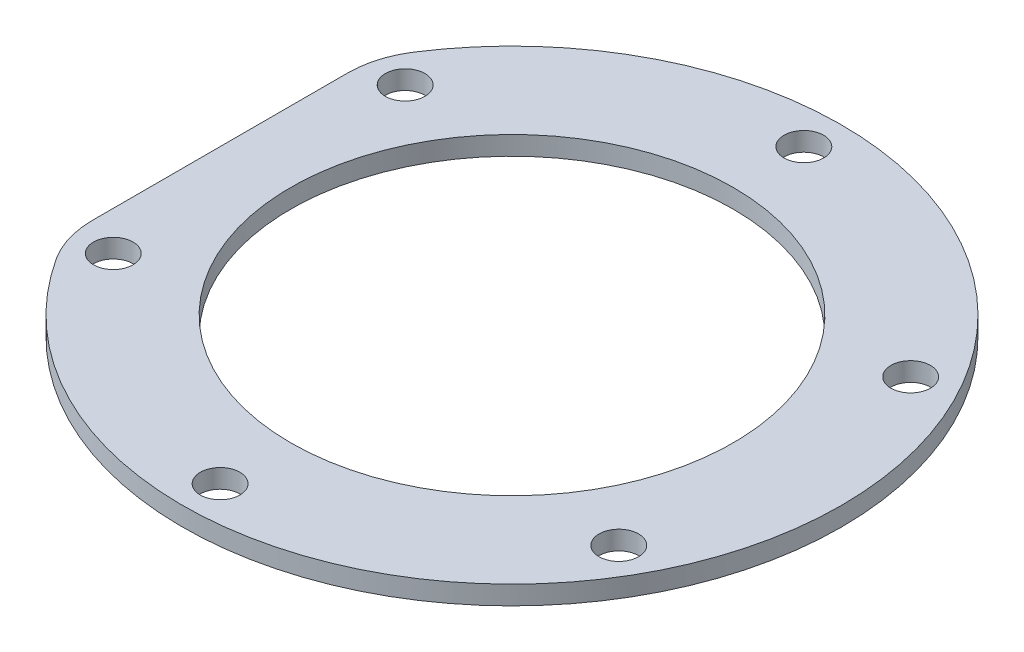
from build123d import *

# Parameters (mm, degrees)
SKETCH_1_R      = 23.5
SKETCH_1_R_2    = 2.1
EXTRUDE_1_DEPTH = 2


with BuildPart() as part:
    # 草图1 → 凸台-拉伸1 (new body)
    with BuildSketch(Plane(origin=(0, 0, 0), x_dir=(1, 0, 0), z_dir=(0, 1, 0))):
        with BuildLine():
            Line((-31, -13.564659966), (-31, 13.564659966))
            ThreePointArc((-31, 13.564659966), (-30.591663047, 16.393087091), (-29.4, 18.990523953))
            ThreePointArc((-29.4, 18.990523953), (35, 0), (-29.4, -18.990523953))
            ThreePointArc((-29.4, -18.990523953), (-30.591663047, -16.393087091), (-31, -13.564659966))
        make_face()
        with Locations(Location((0, 0, 0), (0, 0, 270))):
            Circle(SKETCH_1_R, mode=Mode.SUBTRACT)
        with Locations(Location((0, 31, 0), (0, 0, 270))):
            Circle(SKETCH_1_R_2, mode=Mode.SUBTRACT)
        with Locations(Location((26.846787517, 15.5, 0), (0, 0, 270))):
            Circle(SKETCH_1_R_2, mode=Mode.SUBTRACT)
        with Locations(Location((26.846787517, -15.5, 0), (0, 0, 270))):
            Circle(SKETCH_1_R_2, mode=Mode.SUBTRACT)
        with Locations(Location((0, -31, 0), (0, 0, 270))):
            Circle(SKETCH_1_R_2, mode=Mode.SUBTRACT)
        with Locations(Location((-26.846787517, -15.5, 0), (0, 0, 270))):
            Circle(SKETCH_1_R_2, mode=Mode.SUBTRACT)
        with Locations(Location((-26.846787517, 15.5, 0), (0, 0, 270))):
            Circle(SKETCH_1_R_2, mode=Mode.SUBTRACT)
    extrude(amount=EXTRUDE_1_DEPTH)


solid = part.part
